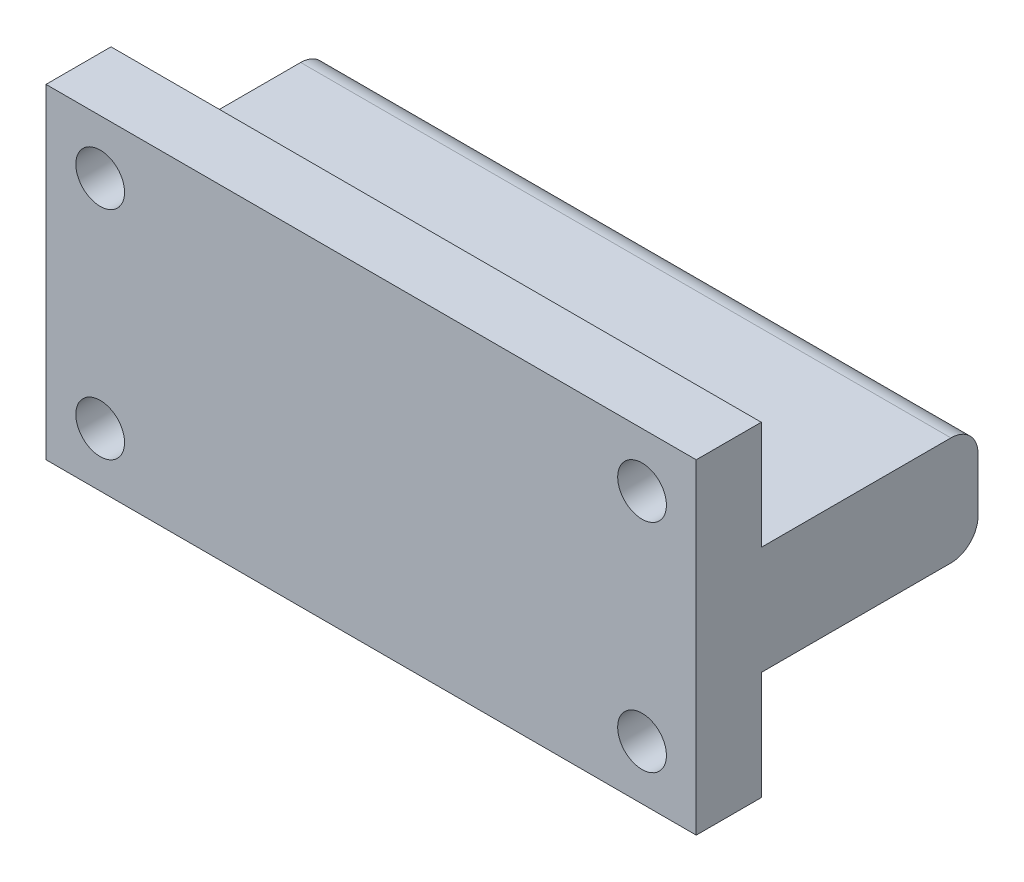
from build123d import *

# Parameters (mm, degrees)
SKETCH1_W                = 120
SKETCH1_H                = 60
BOSS_EXTRUDE1_DEPTH      = 12
M6_CLEARANCE_HOLE1_D     = 9
M6_CLEARANCE_HOLE1_DEPTH = 32.75
M6_CLEARANCE_HOLE1_TIP   = 2.703872786
SKETCH3_W                = 120
SKETCH3_H                = 20
BOSS_EXTRUDE2_DEPTH      = 40
FILLET1_R                = 5


with BuildPart() as part:
    # Sketch1 → Boss-Extrude1 (new body)
    with BuildSketch(Plane.XY):
        with Locations((60, 30)):
            Rectangle(SKETCH1_W, SKETCH1_H)
    extrude(amount=BOSS_EXTRUDE1_DEPTH)

    # M6 Clearance Hole1
    with Locations(Plane(origin=(0, 0, 0), x_dir=(-1, 0, 0), z_dir=(0, 0, -1))):
        with Locations((-110, 50), (-10, 50), (-10, 10), (-110, 10)):
            Hole(M6_CLEARANCE_HOLE1_D / 2, depth=M6_CLEARANCE_HOLE1_DEPTH)
            with Locations((0, 0, -(M6_CLEARANCE_HOLE1_DEPTH + M6_CLEARANCE_HOLE1_TIP / 2))):  # 118° drill point
                Cone(0, M6_CLEARANCE_HOLE1_D / 2, M6_CLEARANCE_HOLE1_TIP, mode=Mode.SUBTRACT)

    # Sketch3 → Boss-Extrude2 (add)
    with BuildSketch(Plane.XY):
        with Locations((60, 30)):
            Rectangle(SKETCH3_W, SKETCH3_H)
    extrude(amount=-BOSS_EXTRUDE2_DEPTH)

    # Fillet1
    fillet1_edges = [part.edges().sort_by_distance(p)[0] for p in [
        (60, 20, -40),
        (60, 40, -40),
    ]]
    fillet(fillet1_edges, radius=FILLET1_R)


solid = part.part
